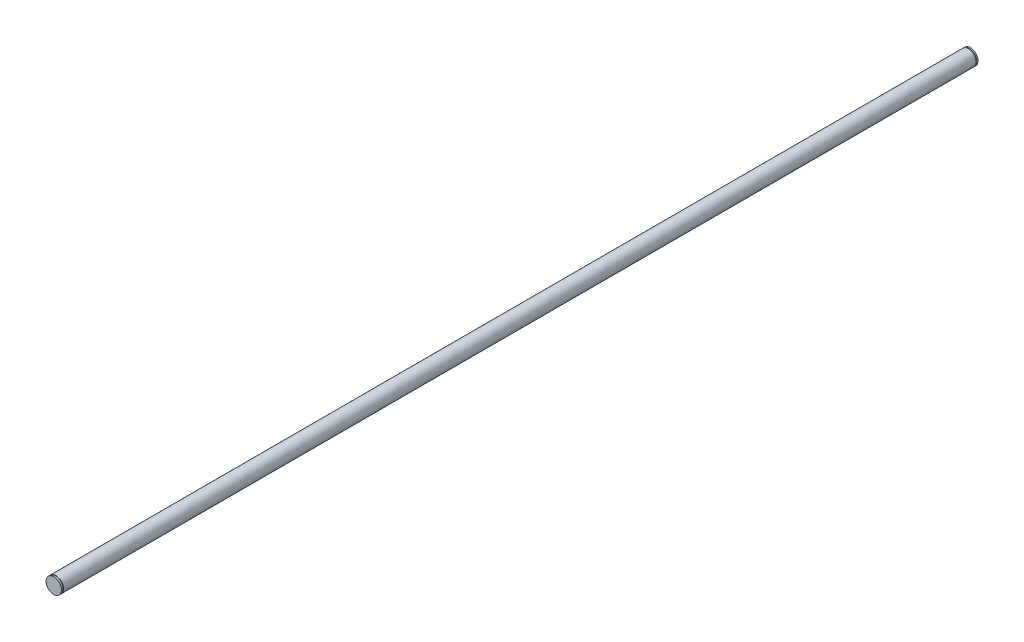
from build123d import *

# Parameters (mm, degrees)
SKETCH_1_R          = 12.5
EXTRUDE_1_DEPTH     = 1470
EXTRUDE_START       = 50
SKETCH_9_R          = 12.5
EXTRUDE_5_DEPTH     = 50
SKETCH_2_W          = 0.55
SKETCH_2_H          = 1.3
CUT_EXTRUDE_START   = -16.5
SKETCH_11_R         = 12.5
CUT_EXTRUDE_2_DEPTH = 16.5
SKETCH_12_R         = 12.5
CUT_EXTRUDE_3_DEPTH = 16.5


with BuildPart() as part:
    # 草图1 → 凸台-拉伸1 (new body)
    with BuildSketch(Plane.XY):
        Circle(SKETCH_1_R)
    extrude(amount=EXTRUDE_1_DEPTH)

    # 草图9 → 凸台-拉伸5 (add)
    with BuildSketch(Plane(origin=(0, 0, 0), x_dir=(-1, 0, 0), z_dir=(0, 0, -1)).offset(EXTRUDE_START)):
        Circle(SKETCH_9_R)
    extrude(amount=-EXTRUDE_5_DEPTH)

    # 草图2 → 切除-旋转1 (revolve, cut)
    with BuildSketch(Plane(origin=(0, 0, 0), x_dir=(1, 0, 0), z_dir=(0, 1, 0)), mode=Mode.PRIVATE) as cut_revolve_1_sk:
        with Locations((12.225, -1450.65)):
            Rectangle(SKETCH_2_W, SKETCH_2_H)
        with Locations((-12.225, -1450.65)):
            Rectangle(SKETCH_2_W, SKETCH_2_H)
        with Locations((-12.225, 30.65)):
            Rectangle(SKETCH_2_W, SKETCH_2_H)
        with Locations((12.225, 30.65)):
            Rectangle(SKETCH_2_W, SKETCH_2_H)
    revolve(cut_revolve_1_sk.sketch.rotate(Axis((0, 0, 1476.033406801), (0, 0, 1)), 180), axis=Axis((0, 0, 1476.033406801), (0, 0, 1)), mode=Mode.SUBTRACT)

    # 草图11 → 切除-拉伸2 (cut)
    with BuildSketch(Plane.XY.offset(1470).offset(CUT_EXTRUDE_START)):
        with Locations(Location((0, 0, 0), (0, 0, 180))):
            Circle(SKETCH_11_R)
    extrude(amount=CUT_EXTRUDE_2_DEPTH, mode=Mode.SUBTRACT)

    # 草图12 → 切除-拉伸3 (cut)
    with BuildSketch(Plane(origin=(0, 0, -50), x_dir=(-1, 0, 0), z_dir=(0, 0, -1))):
        Circle(SKETCH_12_R)
    extrude(amount=-CUT_EXTRUDE_3_DEPTH, mode=Mode.SUBTRACT)


solid = part.part
